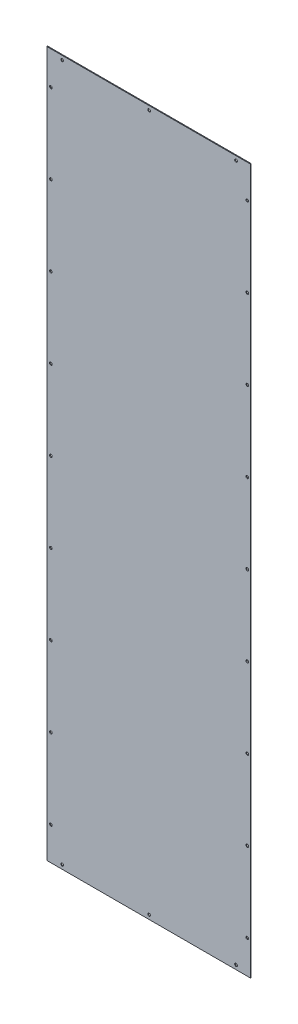
from build123d import *

# Parameters (mm, degrees)
SKETCH_1_W          = 494.5
SKETCH_1_H          = 1703
SKETCH_1_R          = 3.25
EXTRUDE_1_DEPTH     = 2
SKETCH_2_W          = 2.5
SKETCH_2_H          = 2
CUT_EXTRUDE_1_DEPTH = 1721.856055137


with BuildPart() as part:
    # 草图1 → 凸台-拉伸1 (new body)
    with BuildSketch(Plane.XY):
        Rectangle(SKETCH_1_W, SKETCH_1_H)
        with Locations((-237.25, 0)):
            Circle(SKETCH_1_R, mode=Mode.SUBTRACT)
        with Locations((-237.25, -192.875)):
            Circle(SKETCH_1_R, mode=Mode.SUBTRACT)
        with Locations((-237.25, -385.75)):
            Circle(SKETCH_1_R, mode=Mode.SUBTRACT)
        with Locations((-237.25, -578.625)):
            Circle(SKETCH_1_R, mode=Mode.SUBTRACT)
        with Locations((-237.25, -771.5)):
            Circle(SKETCH_1_R, mode=Mode.SUBTRACT)
        with Locations((0, -841.5)):
            Circle(SKETCH_1_R, mode=Mode.SUBTRACT)
        with Locations(Location((0, 841.5, 0), (0, 0, 180))):
            Circle(SKETCH_1_R, mode=Mode.SUBTRACT)
        with Locations(Location((-237.25, 771.5, 0), (0, 0, 180))):
            Circle(SKETCH_1_R, mode=Mode.SUBTRACT)
        with Locations(Location((-237.25, 578.625, 0), (0, 0, 180))):
            Circle(SKETCH_1_R, mode=Mode.SUBTRACT)
        with Locations(Location((-237.25, 385.75, 0), (0, 0, 180))):
            Circle(SKETCH_1_R, mode=Mode.SUBTRACT)
        with Locations(Location((-237.25, 192.875, 0), (0, 0, 180))):
            Circle(SKETCH_1_R, mode=Mode.SUBTRACT)
        with Locations((237.25, 192.875)):
            Circle(SKETCH_1_R, mode=Mode.SUBTRACT)
        with Locations((237.25, 385.75)):
            Circle(SKETCH_1_R, mode=Mode.SUBTRACT)
        with Locations((237.25, 578.625)):
            Circle(SKETCH_1_R, mode=Mode.SUBTRACT)
        with Locations((237.25, 771.5)):
            Circle(SKETCH_1_R, mode=Mode.SUBTRACT)
        with Locations(Location((237.25, -771.5, 0), (0, 0, 180))):
            Circle(SKETCH_1_R, mode=Mode.SUBTRACT)
        with Locations(Location((237.25, -578.625, 0), (0, 0, 180))):
            Circle(SKETCH_1_R, mode=Mode.SUBTRACT)
        with Locations(Location((237.25, -385.75, 0), (0, 0, 180))):
            Circle(SKETCH_1_R, mode=Mode.SUBTRACT)
        with Locations(Location((237.25, -192.875, 0), (0, 0, 180))):
            Circle(SKETCH_1_R, mode=Mode.SUBTRACT)
        with Locations(Location((237.25, 0, 0), (0, 0, 180))):
            Circle(SKETCH_1_R, mode=Mode.SUBTRACT)
        with Locations((-210, 841.5)):
            Circle(SKETCH_1_R, mode=Mode.SUBTRACT)
        with Locations((210, 841.5)):
            Circle(SKETCH_1_R, mode=Mode.SUBTRACT)
        with Locations(Location((-210, -841.5, 0), (0, 0, 180))):
            Circle(SKETCH_1_R, mode=Mode.SUBTRACT)
        with Locations(Location((210, -841.5, 0), (0, 0, 180))):
            Circle(SKETCH_1_R, mode=Mode.SUBTRACT)
    extrude(amount=EXTRUDE_1_DEPTH)

    # 草图2 → 切除-拉伸1 (cut, through all)
    with BuildSketch(Plane(origin=(0, -851.5, 0), x_dir=(-1, 0, 0), z_dir=(0, -1, 0))):
        with Locations((-246, -1)):
            Rectangle(SKETCH_2_W, SKETCH_2_H)
    extrude(amount=-CUT_EXTRUDE_1_DEPTH, mode=Mode.SUBTRACT)


solid = part.part
